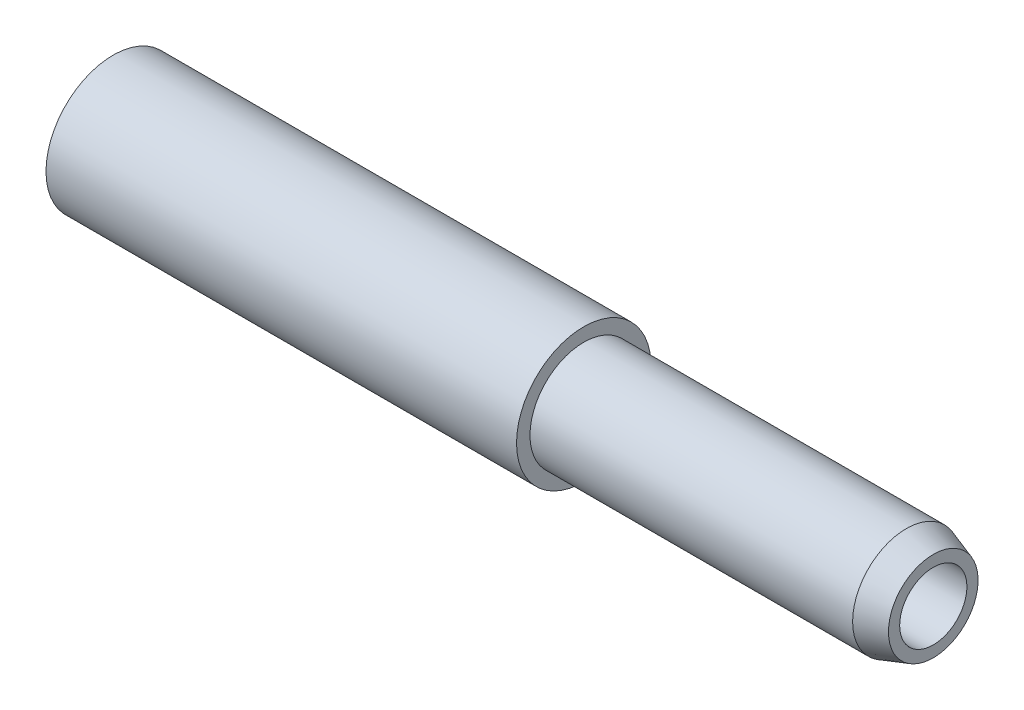
from build123d import *

# Parameters (mm, degrees)
CHAMFER1_SIZE  = 2
CHAMFER1_SIZE2 = 6


with BuildPart() as part:
    # Sketch1 → Revolve1 (revolve)
    with BuildSketch(Plane.XY, mode=Mode.PRIVATE) as revolve1_sk:
        Polygon((0, 7.5), (0, 15), (105, 15), (105, 12), (183, 12), (183, 7.5), (33, 7.5), (33, 3.25), (8, 3.25), (8, 7.5), align=None)
    revolve(revolve1_sk.sketch.rotate(Axis((0, 0, 0), (1, 0, 0)), 90), axis=Axis((0, 0, 0), (1, 0, 0)))

    # Chamfer1
    chamfer1_edges = [part.edges().sort_by_distance(p)[0] for p in [
        (183, 0, -12),
    ]]
    chamfer1_side = [part.faces().sort_by_distance(p)[0] for p in [
        (183, 0, -11.660588745),
    ]]
    chamfer(chamfer1_edges, length=CHAMFER1_SIZE, length2=CHAMFER1_SIZE2, reference=chamfer1_side[0])


solid = part.part
